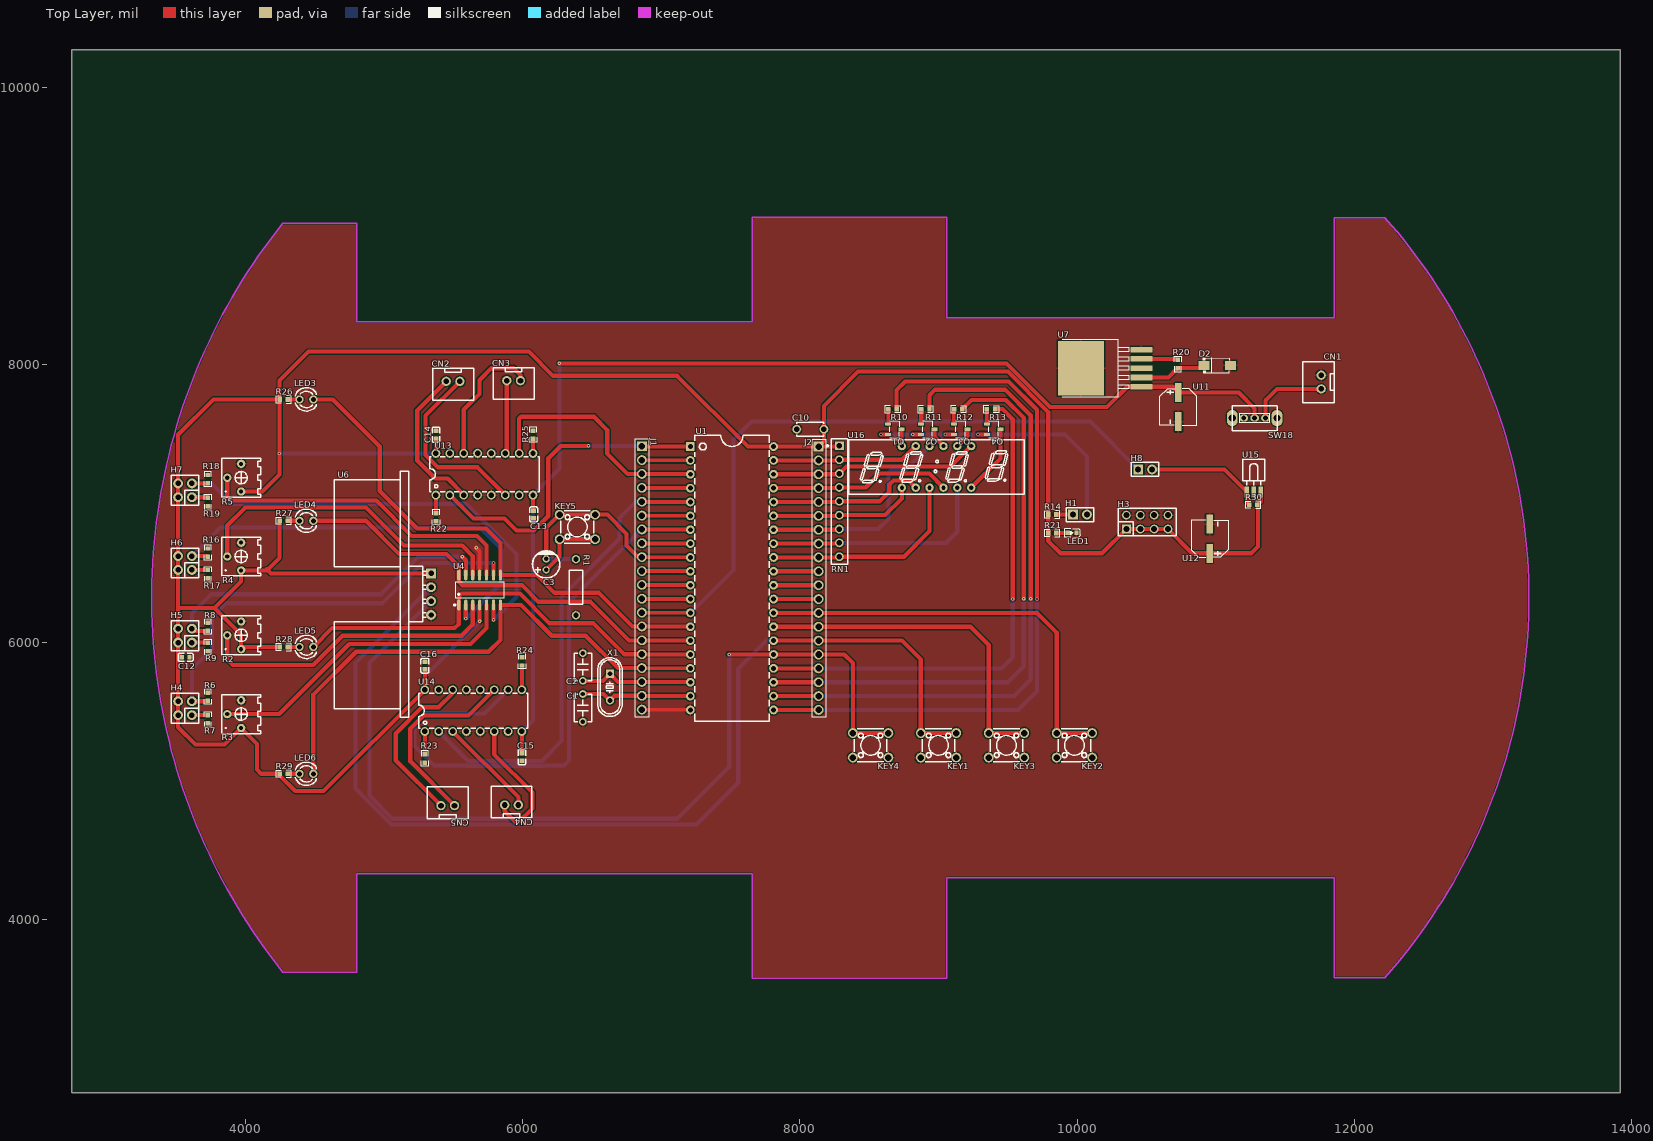
[diagram p0: Top Layer view]
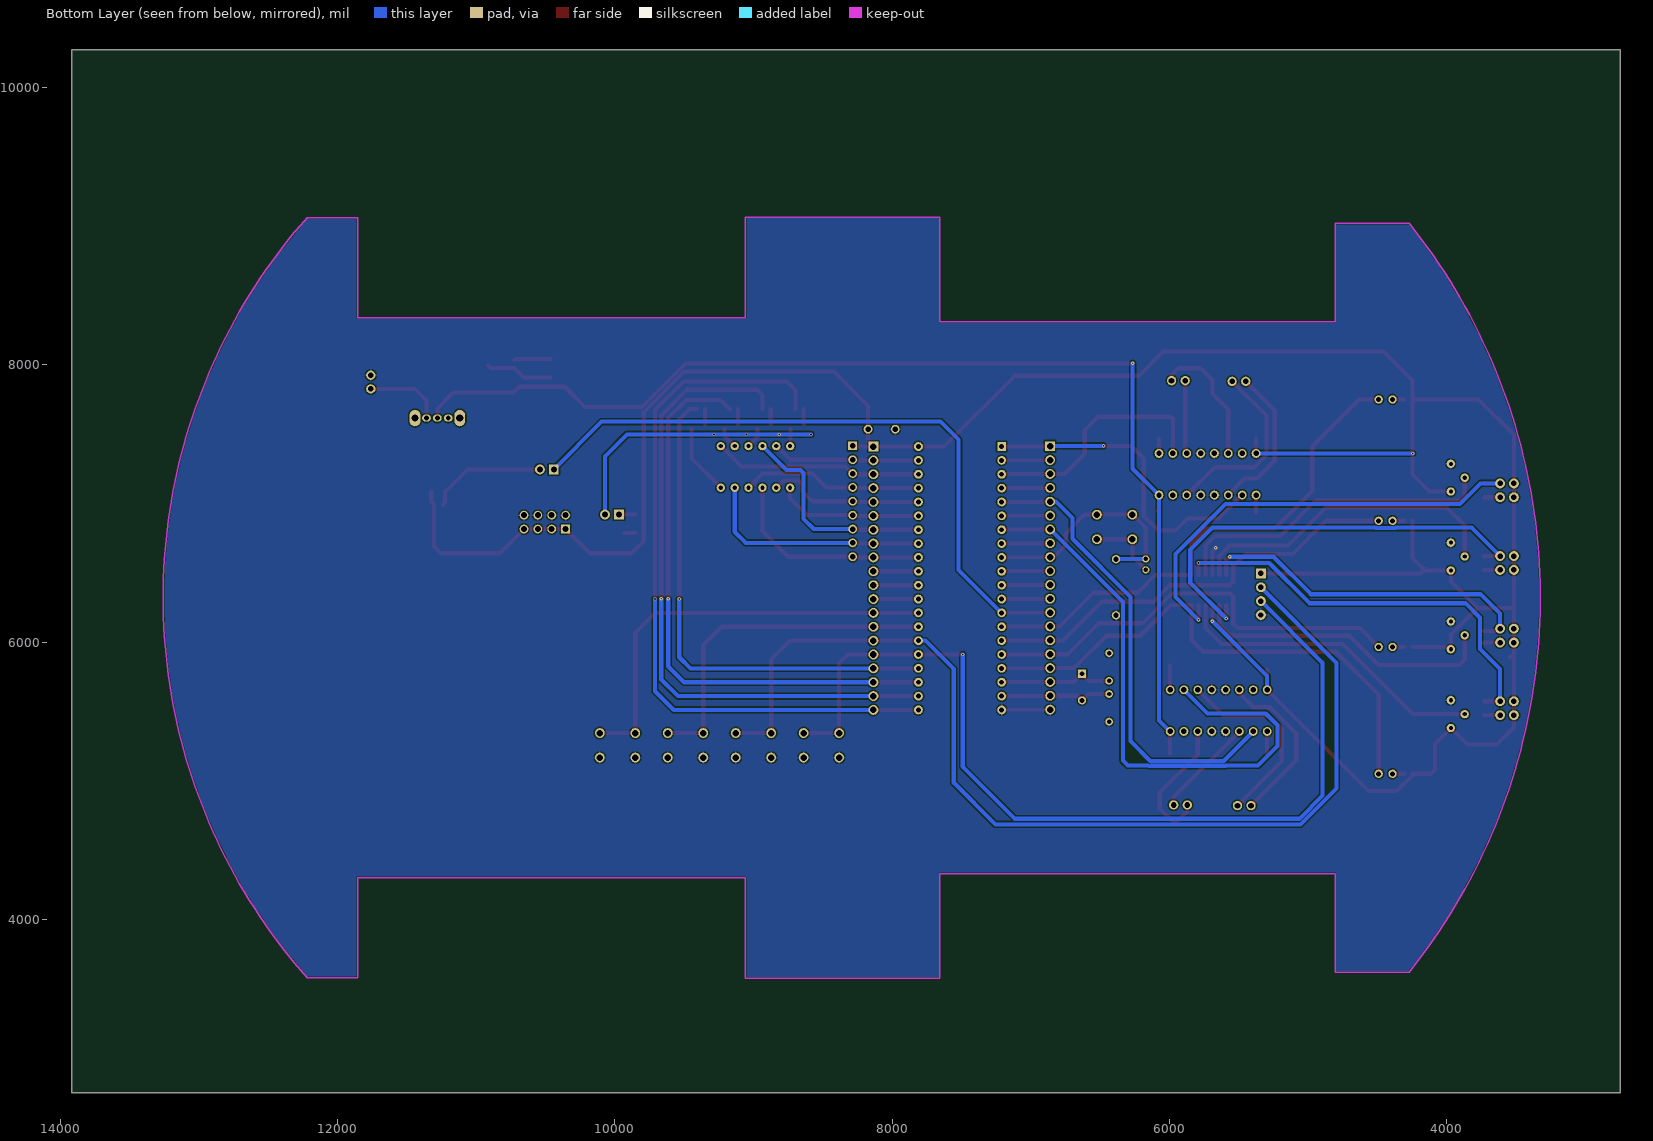
[diagram p1: Bottom Layer view, seen from below]
# Altium PCB MISC51732.pcbdoc
Units mil, origin at the board's own origin, x right, y up, seen from the top; angles counter-clockwise.
Board outline 11165 x 7520 mil, 2 copper layers (Top Layer, Bottom Layer), stack 62.206 mil thick; 80 components, 94 nets, 333 pads, 18 vias.

## Layer stack, top to bottom
Top Solder Mask Layer: solder mask 0.394, Dk 3.3
Top Layer: signal copper 1.379
Dielectric1: surface 59.449, FR4, Dk 4.5
Bottom Layer: signal copper 1.378
Bottom Solder Mask Layer: solder mask 0.394, Dk 3.3

## Board outline
13915,2750 2750,2750 2750,10270 13915,10270

## Design rules (kind name [scope] priority, off if disabled: settings)
BoardOutlineClearance copperThickness2oz_1 [All] p2 off: genericclearance=7.99 ignorepadtopadclearanceinfootprint=FALSE except(0: Arc-SplitContinuation Track-SplitContinuation SMDPad-SplitContinuation THPad-SplitContinuation Via-SplitContinuation Fill-SplitContinuation Region-SplitContinuation Poly-SplitContinuation Text-SplitContinuation Hole-SplitContinuation; 5.98: Arc-CutoutEdge SMDPad-CutoutEdge THPad-CutoutEdge Via-CutoutEdge Fill-CutoutEdge Region-CutoutEdge Text-CutoutEdge; 6.93: Hole-OutlineEdge Hole-CutoutEdge; 10: Poly-OutlineEdge Poly-CutoutEdge; 11.81: Arc-OutlineEdge Track-OutlineEdge SMDPad-OutlineEdge THPad-OutlineEdge Via-OutlineEdge Fill-OutlineEdge Region-OutlineEdge Text-OutlineEdge Track-CutoutEdge)
BoardOutlineClearance copperThickness1oz_1 [All] p4: genericclearance=4.02 ignorepadtopadclearanceinfootprint=FALSE except(0: Arc-SplitContinuation Track-SplitContinuation SMDPad-SplitContinuation THPad-SplitContinuation Via-SplitContinuation Fill-SplitContinuation Region-SplitContinuation Poly-SplitContinuation Text-SplitContinuation Hole-SplitContinuation; 6: SMDPad-CutoutEdge THPad-CutoutEdge Via-CutoutEdge Fill-CutoutEdge Region-CutoutEdge Text-CutoutEdge; 6.93: Hole-OutlineEdge Hole-CutoutEdge; 10: Poly-OutlineEdge Poly-CutoutEdge; 11.8: Arc-OutlineEdge Track-OutlineEdge SMDPad-OutlineEdge THPad-OutlineEdge Via-OutlineEdge Fill-OutlineEdge Region-OutlineEdge Text-OutlineEdge; 11.81: Arc-CutoutEdge Track-CutoutEdge)
Clearance copperThickness2oz [All] p1 off: gap=7.99 ignorepadtopadclearanceinfootprint=FALSE except(5.98: SMDPad-Track SMDPad-SMDPad THPad-Track SMDPad-THPad THPad-THPad Track-Via SMDPad-Via THPad-Via Via-Via Fill-Track Region-Track Fill-SMDPad Region-SMDPad Fill-THPad Region-THPad Fill-Via Region-Via Fill-Fill Fill-Region Region-Region Arc-Track Arc-SMDPad Arc-THPad Arc-Via Fill-Arc Region-Arc Arc-Arc Text-Track SMDPad-Text Text-THPad Text-Via Fill-Text Region-Text Arc-Text Text-Text; 6.93: Hole-Track Hole-SMDPad Hole-THPad Hole-Via Fill-Hole Region-Hole Hole-Arc Hole-Text; 10: Poly-Track Poly-SMDPad Poly-THPad Poly-Via Poly-Fill Poly-Region Poly-Poly Poly-Arc Poly-Text Poly-Hole)
Clearance copperThickness1oz [All] p3: gap=4.02 ignorepadtopadclearanceinfootprint=FALSE except(5.98: SMDPad-Track SMDPad-SMDPad THPad-Track SMDPad-THPad THPad-THPad Track-Via SMDPad-Via THPad-Via Via-Via Fill-Track Region-Track Fill-SMDPad Region-SMDPad Fill-THPad Region-THPad Fill-Via Region-Via Fill-Fill Fill-Region Region-Region; 6: Arc-Track Arc-SMDPad Arc-THPad Arc-Via Fill-Arc Region-Arc Arc-Arc Text-Track SMDPad-Text Text-THPad Text-Via Fill-Text Region-Text Arc-Text Text-Text; 6.93: Hole-Track Hole-SMDPad Hole-THPad Hole-Via Fill-Hole Region-Hole Hole-Arc Hole-Text; 10: Poly-Track Poly-SMDPad Poly-THPad Poly-Via Poly-Fill Poly-Region Poly-Poly Poly-Arc Poly-Text Poly-Hole)
DiffPairsRouting differentialPair [All] p1: maxlimit=6 minlimit=6 mostfreqgap=6 toplayer_minwidth=5 toplayer_prefwidth=10 toplayer_maxwidth=100 toplayer_mingap=6 toplayer_prefgap=6 toplayer_maxgap=6 bottomlayer_minwidth=5 bottomlayer_prefwidth=10 bottomlayer_maxwidth=100 bottomlayer_mingap=6 bottomlayer_prefgap=6 bottomlayer_maxgap=6 maxuncoupledlength=10
HoleToHoleClearance otherClearance [All] p1: gap=11.81 allowstackedmicrovias=TRUE
Length netLength [All] p1: minlimit=0 maxlimit=0
MatchedLengths netLengthTolerance [All] p1: tolerance=1000
PasteMaskExpansion pasteMaskExpansion [All] p1: expansion=0
PlaneConnect innerPlane [All] p1: planeconnectstyle=Relief reliefexpansion=20 reliefentries=4 reliefconductorwidth=10 reliefairgap=10
PolygonConnect copperRegion [(InNet('GND'))] p1: connectstyle=Relief reliefconductorwidth=10 reliefentries=4 polygonreliefangle="90 Angle" airgapwidth=10 via.connectstyle=Relief via.reliefconductorwidth=10 via.reliefentries=4 via.polygonreliefangle="90 Angle" via.airgapwidth=10
RoutingVias viaSize [All] p1: holewidth=12.01 width=24.02 viastyle="Through Hole" minholewidth=11.81 minwidth=19.68 maxholewidth=248.03 maxwidth=393.7
SolderMaskExpansion solderMaskExpansion [IsVia] p1: expansion=-1000 istentingtop=TRUE
SolderMaskExpansion solderMaskExpansion [All] p2: expansion=2 istentingtop=FALSE
Width copperThickness2oz_2 [All] p1 off: maxlimit=100 minlimit=8 preferedwidth=10
Width copperThickness1oz_2 [All] p2: maxlimit=100 minlimit=5 preferedwidth=10

## Components (designator, comment, footprint, x,y, rotation, side; value= is the part's Value field where it differs from the comment)
C1 "" CAP-TH_L5.0-W2.5-P5.08-D0.7 6435,5525 r270 top
C2 "" CAP-TH_L5.0-W2.5-P5.08-D0.7 6435,5820 r90 top
C3 "" CAP-TH_BD5.0-P2.00-D0.8-FD 6170,6560 r90 top
C10 "" CAP-TH_L5.0-W2.5-P5.00-D1.0 8075,7535 r0 top
C12 "104" C0603 3570,5890 r0 top
C13 "100nF" C0603 6080,6920 r270 top
C14 "100nF" C0603 5375,7495 r90 top
C15 "100nF" C0603 5995,5170 r270 top
C16 "100nF" C0603 5295,5830 r90 top
CN1 "XH2.54*2P_through-hole" CONN-TH_2P-P2.50-XH2.54-2P 11760,7875 r270 top
CN2 "XH2.54*2P_through-hole" CONN-TH_2P-P2.50-XH2.54-2P 5498.36,7880.12 r0 top
CN3 "XH2.54*2P_through-hole" CONN-TH_2P-P2.50-XH2.54-2P 5935,7885 r0 top
CN4 "XH2.54*2P_through-hole" CONN-TH_2P-P2.50-XH2.54-2P 5920,4825 r180 top
CN5 "XH2.54*2P_through-hole" CONN-TH_2P-P2.50-XH2.54-2P 5460,4820 r180 top
D2 "SS34" SMA_L4.3-W2.6-LS5.0-RD 11010,7995 r0 top
H1 "" HDR-TH_2P-P2.54-V-M-1 10020.44,6919.23 r0 top
H3 "" HDR-TH_8P-P2.54-V-F-R2-C4-S2.54-1 10505,6865 r0 top
H4 "" HDR-TH_4P-P2.54-V-F-R2-C2-S2.54 3564.9,5522.49 r90 top
H5 "" HDR-TH_4P-P2.54-V-F-R2-C2-S2.54 3564.9,6046.36 r90 top
H6 "" HDR-TH_4P-P2.54-V-F-R2-C2-S2.54 3564.9,6570.23 r90 top
H7 "" HDR-TH_4P-P2.54-V-F-R2-C2-S2.54 3564.9,7094.1 r90 top
H8 "" HDR-TH_2P-P2.54-V-M-1 10490,7245 r0 top
J1 "" HDR-TH_20P-P2.54-V-M-1 6860.16,6462.19 r270 top
J2 "" HDR-TH_20P-P2.54-V-M-1 8135,6460 r270 top
KEY1 "UK-B0202-G5-160" SW-TH_4P-L6.0-W6.0-P4.50-LS6.5 9000,5255 r180 top
KEY2 "UK-B0202-G5-160" SW-TH_4P-L6.0-W6.0-P4.50-LS6.5 9980,5255 r180 top
KEY3 "UK-B0202-G5-160" SW-TH_4P-L6.0-W6.0-P4.50-LS6.5 9490,5255 r180 top
KEY4 "UK-B0202-G5-160" SW-TH_4P-L6.0-W6.0-P4.50-LS6.5 8510,5255 r180 top
KEY5 "UK-B0202-G5-160" SW-TH_4P-L6.0-W6.0-P4.50-LS6.5 6395,6830 r0 top
LED1 "" LED_0603 9961.23,6786.73 r180 top
LED3 "" LED-TH_BD3.0-P2.54-FD 4440.51,7749.41 r0 top
LED4 "" LED-TH_BD3.0-P2.54-FD 4440.51,6874.41 r0 top
LED5 "" LED-TH_BD3.0-P2.54-FD 4440.51,5964.41 r0 top
LED6 "" LED-TH_BD3.0-P2.54-FD 4440.51,5049.41 r0 top
Q1 "S8550" SOT-23-3_L2.9-W1.6-P1.90-LS2.8-BR 8683.19,7534.47 r180 top
Q2 "S8550" SOT-23-3_L2.9-W1.6-P1.90-LS2.8-BR 8921.41,7534.47 r180 top
Q3 "S8550" SOT-23-3_L2.9-W1.6-P1.90-LS2.8-BR 9159.63,7534.47 r180 top
Q4 "S8550" SOT-23-3_L2.9-W1.6-P1.90-LS2.8-BR 9397.84,7534.47 r180 top
R1 "" RES-TH_BD2.4-L6.3-P10.30-D0.6 6385,6395 r270 top
R2 "-" RES-ADJ-TH_3362P 3920,6048.33 r90 top
R3 "-" RES-ADJ-TH_3362P 3920,5480 r90 top
R4 "-" RES-ADJ-TH_3362P 3920,6616.67 r90 top
R5 "-" RES-ADJ-TH_3362P 3920,7185 r90 top
R6 "10K" R0603 3730,5605 r90 top
R7 "100" R0603 3730,5442.91 r270 top
R8 "10K" R0603 3730,6110 r90 top
R9 "100" R0603 3730,5965 r270 top
R10 "1K" R0603 8668.19,7679.47 r180 top
R11 "1K" R0603 8904.89,7679.47 r180 top
R12 "1K" R0603 9141.59,7679.47 r180 top
R13 "1K" R0603 9378.29,7679.47 r180 top
R14 "33" R0603 9820,6920 r0 top
R16 "10K" R0603 3730,6645 r90 top
R17 "100" R0603 3730,6490 r270 top
R18 "10K" R0603 3730,7175 r90 top
R19 "100" R0603 3730,7010 r270 top
R20 "33U" R0603 10725,8005 r270 top
R21 "2K" R0603 9820.46,6786.73 r0 top
R22 "1K" R0603 5375,6900 r90 top
R23 "1K" R0603 5295,5160 r90 top
R24 "1K" R0603 5995,5860 r90 top
R25 "1K" R0603 6075,7495 r90 top
R26 "1K" R0603 4277.03,7749.41 r0 top
R27 "1K" R0603 4277.03,6874.41 r0 top
R28 "1K" R0603 4277.03,5964.41 r0 top
R29 "1K" R0603 4277.03,5049.41 r0 top
R30 "10K" R0603 11270,6990 r0 top
RN1 "" RES-ARRAY-TH_9P-P2.54-D1.0 8285,7015 r270 top
SW18 "" 拨动开关 11285,7615 r180 top
U1 "" DIP-40_L52.0-W13.7-P2.54-LS15.2-BL 7510,6460 r270 top
U4 "LM324NLM324" SOP-14_L8.6-W3.9-P1.27-LS6.0-BL 5690,6375 r0 top
U6 "HC-SR04" TH_HC-SR04V 5340,6345 r270 top
U7 "LM2596SX-5.0/NOPB-YJLTY" TO-263-5_L10.0-W8.4-P1.70-LS15.3-BR 10245,7975 r0 top
U11 "220uF" CAP-SMD_BD6.3-L6.6-W6.6-LS7.2-FD 10730,7695 r270 top
U12 "220uF" CAP-SMD_BD6.3-L6.6-W6.6-LS7.2-FD 10955.02,6745 r90 top
U13 "L293D" DIP-16_L20.0-W6.4-P2.54-LS7.6-BL 5725,7210 r0 top
U14 "L293D" DIP-16_L20.0-W6.4-P2.54-LS7.6-BL 5645,5505 r0 top
U15 "CH0038A_38B/5*5mm/infrared receiver" OPTO-SMD_CH0038A_38B 11273.63,7083.36 r0 top
U16 "0.28 4-digit display" LED-SEG-TH_12P-L32.1-W10.0-P12.7-S7.62-BL 8985.44,7262.93 r0 top
X1 "" HC-49US_L11.5-W4.5-P4.88 6630,5675 r270 top

## Footprints (in the part's own frame and the unit in brackets; to place one, negate y for a bottom-side part, rotate by r counter-clockwise, add the part's x,y. Pads: shape width x height; smd on the part's side, far side on the other; paste and mask are expansions set on the pad)
C0603 [mm]
  rect 0.8x0.9 smd: 1(-0.7,0) 2(0.7,0)
  silkscreen extent -1.39,-0.71 1.39,0.71
CAP-SMD_BD6.3-L6.6-W6.6-LS7.2-FD [mm]
  rect 3.5x1.2 smd: 1(-2.67,0) 2(2.67,0)
  silkscreen extent -3.38,-3.38 3.38,3.38
CAP-TH_BD5.0-P2.00-D0.8-FD [mil]
  round 51.2 hole 31.5 paste+0 mask+2: 1(-39.4,0) 2(39.4,0)
  silkscreen extent -98,-98 98,98
CAP-TH_L5.0-W2.5-P5.00-D1.0 [mil]
  round 63 hole 39.4 paste+0 mask+2: 1(-98.4,0) 2(98.4,0)
  silkscreen extent -98,-50 98,49
CAP-TH_L5.0-W2.5-P5.08-D0.7 [mm]
  round 1.4 hole 0.8 paste+0 mask+0.051: 1(-2.54,0) 2(2.54,0)
  silkscreen extent -2.54,-1.59 2.54,1.59
CONN-TH_2P-P2.50-XH2.54-2P [mm]
  round 1.7 hole 1.05 paste+0 mask+0.05: 1(1.25,0) 2(-1.25,0)
  silkscreen extent -3.75,-3.42 3.75,2.37
DIP-16_L20.0-W6.4-P2.54-LS7.6-BL [mm]
  round 1.6 hole 1: 1(-8.89,-3.81) 2(-6.35,-3.81) 3(-3.81,-3.81) 4(-1.27,-3.81) 5(1.27,-3.81) 6(3.81,-3.81) 7(6.35,-3.81) 8(8.89,-3.81) 9(8.89,3.81) 10(6.35,3.81) 11(3.81,3.81) 12(1.27,3.81) 13(-1.27,3.81) 14(-3.81,3.81) 15(-6.35,3.81) 16(-8.89,3.81)
  silkscreen extent -10,-3.2 10,3.2
DIP-40_L52.0-W13.7-P2.54-LS15.2-BL [mil]
  rect 63x63 hole 35 paste+0 mask+2: 1(-950,-300)
  round 63 hole 35 paste+0 mask+2: 2(-850,-300) 3(-750,-300) 4(-650,-300) 5(-550,-300) 6(-450,-300) 7(-350,-300) 8(-250,-300) 9(-150,-300) 10(-50,-300) 11(50,-300) 12(150,-300) 13(250,-300) 14(350,-300) 15(450,-300) 16(550,-300) 17(650,-300) 18(750,-300) 19(850,-300) 20(950,-300) 21(950,300) 22(850,300) 23(750,300) 24(650,300) 25(550,300) 26(450,300) 27(350,300) 28(250,300) 29(150,300) 30(50,300) 31(-50,300) 32(-150,300) 33(-250,300) 34(-350,300) 35(-450,300) 36(-550,300) 37(-650,300) 38(-750,300) 39(-850,300) 40(-950,300)
  silkscreen extent -1030,-270 1030,270
HC-49US_L11.5-W4.5-P4.88 [mil]
  rect 59.1x59.1 hole 35.4 paste+0 mask+2: 1(-96.1,0)
  round 59.1 hole 35.4 paste+0 mask+2: 2(96.1,0)
  silkscreen extent -212,-89 212,89
HDR-TH_2P-P2.54-V-M-1 [mm]
  rect 1.8x1.8 hole 1.1: 1(-1.27,0)
  round 1.8 hole 1.1: 2(1.27,0)
  silkscreen extent -2.54,-1.27 2.54,1.27
HDR-TH_4P-P2.54-V-F-R2-C2-S2.54 [mm]
  round 1.8 hole 1: 1(-1.27,-1.27) 2(-1.27,1.27) 3(1.27,-1.27) 4(1.27,1.27)
  silkscreen extent -2.74,-2.5 2.74,2.5
HDR-TH_8P-P2.54-V-F-R2-C4-S2.54-1 [mm]
  rect 1.6x1.6 hole 1.1: 1(-3.81,-1.27)
  round 1.6 hole 1.1: 2(-3.81,1.27) 3(-1.27,-1.27) 4(-1.27,1.27) 5(1.27,-1.27) 6(1.27,1.27) 7(3.81,-1.27) 8(3.81,1.27)
  silkscreen extent -5.28,-2.5 5.28,2.5
HDR-TH_20P-P2.54-V-M-1 [mil]
  rect 70.9x70.9 hole 47.2 paste+0 mask+2: 1(-950,0)
  round 70.9 hole 47.2 paste+0 mask+2: 2(-850,0) 3(-750,0) 4(-650,0) 5(-550,0) 6(-450,0) 7(-350,0) 8(-250,0) 9(-150,0) 10(-50,0) 11(50,0) 12(150,0) 13(250,0) 14(350,0) 15(450,0) 16(550,0) 17(650,0) 18(750,0) 19(850,0) 20(950,0)
  silkscreen extent -1000,-50 1000,55
LED-SEG-TH_12P-L32.1-W10.0-P12.7-S7.62-BL [mil]
  round 60 hole 30: 1(-250,-150) 2(-150,-150) 3(-50,-150) 4(50,-150) 5(150,-150) 6(250,-150) 7(250,150) 8(150,150) 9(50,150) 10(-50,150) 11(-150,150) 12(-250,150)
  silkscreen extent -634,-197 634,197
LED-TH_BD3.0-P2.54-FD [mil]
  round 60 hole 36 paste+0 mask+2: 1(-50,0) 2(50,0)
  silkscreen extent -81,-84 72,85
LED_0603 [mil]
  rect 31.5x31.5 smd paste+0 mask+2: 1(-33.5,-0.4) 2(29.5,-0.2)
  silkscreen extent -61,-30 53,30
OPTO-SMD_CH0038A_38B [mm]
  rect 0.8x2 smd paste+0 mask+0.05: 1(-1.27,0) 2(0,0) 3(1.27,0)
  silkscreen extent -2,1.23 2,6
R0603 [mil]
  rect 31.75x34.02 smd paste-3937.01 mask+2: 1(-29.66,0) 2(29.66,0)
  silkscreen extent -55,-26 55,26
RES-ADJ-TH_3362P [mil]
  round 60 hole 30: 1(-100,-50) 2(0,50) 3(100,-50)
  silkscreen extent -140,-190 140,90
RES-ARRAY-TH_9P-P2.54-D1.0 [mm]
  rect 1.6x1.6 hole 1 paste+0 mask+0.051: 1(-10.16,0)
  round 1.6 hole 1 paste+0 mask+0.051: 2(-7.62,0) 3(-5.08,0) 4(-2.54,0) 5(0,0) 6(2.54,0) 7(5.08,0) 8(7.62,0) 9(10.16,0)
  silkscreen extent -11.5,-2.31 11.5,1.5
RES-TH_BD2.4-L6.3-P10.30-D0.6 [mil]
  round 60 hole 39.37 paste+0 mask+2: 1(-202.76,0) 2(202.76,0)
  silkscreen extent -124,-47 124,47
SMA_L4.3-W2.6-LS5.0-RD [mm]
  rect 2.046x1.62 smd: 1(-2.404,-0.009) 2(2.404,0.009)
  silkscreen extent -2.61,-1.44 2.16,1.44
SOP-14_L8.6-W3.9-P1.27-LS6.0-BL [mm]
  oval 0.595x1.968 smd: 1(-3.81,-2.734) 2(-2.54,-2.734) 3(-1.27,-2.734) 4(0,-2.734) 5(1.27,-2.734) 6(2.54,-2.734) 7(3.81,-2.734) 8(3.81,2.734) 9(2.54,2.734) 10(1.27,2.734) 11(0,2.734) 12(-1.27,2.734) 13(-2.54,2.734) 14(-3.81,2.734)
  silkscreen extent -4.71,-2.88 4.4,1.52
SOT-23-3_L2.9-W1.6-P1.90-LS2.8-BR [mm]
  rect 1.07x0.6 smd: 1(1.235,-0.95) 2(1.235,0.95) 3(-1.235,0)
  silkscreen extent -0.88,-1.54 0.88,1.54
SW-TH_4P-L6.0-W6.0-P4.50-LS6.5 [mm]
  round 1.8 hole 1.2 paste+0 mask+0.051: 1(-3.25,2.25) 2(3.25,2.25) 3(-3.25,-2.25) 4(3.25,-2.25)
  silkscreen extent -3,-3 3,3
TH_HC-SR04V [mm]
  rect 1.8x1.8 hole 1.001: 1(-3.81,0)
  round 1.8 hole 1.001: 2(-1.27,0) 3(1.27,0) 4(3.81,0)
  silkscreen extent -22.5,-17.7 22.5,-0.89
TO-263-5_L10.0-W8.4-P1.70-LS15.3-BR [mm]
  rect 4x1.02 smd: 1(5.55,-3.4) 2(5.55,-1.7) 3(5.55,0) 4(5.55,1.7) 5(5.55,3.4)
  rect 8.4x10 smd: 6(-5.55,0)
  silkscreen extent -8.91,-5.33 3.2,5.33
拨动开关 [mil]
  oval 63x51.2 hole 35.4 paste+0 mask+2: 1(-73.4,0) 2(5,0) 3(84,0)
  oval 78.7x118.1 hole 51.2 paste+0 mask+2: 4(166.7,0) 5(-156.1,0)
  silkscreen extent -156,-90 167,90

## Via types
v1: diameter 24.02, hole 12, Top Layer to Bottom Layer, 18 vias

## Nets (pads, with @x,y where several pads share a name; then routed paths per layer and width w, separated by ;. In a path a pad name is that pad's centre, name@x,y a point inside that pad or via, vN(x,y) a via of type N, cw(c..) or ccw(c..) an arc to the next point about the centre after c; other vN are vias at no path point)
7.2V: C13.1 C15.1 SW18.2 U7.1 U11.1 U13.8 U14.8 | length 8379.5
  Top Layer w30: C15.1 U14.8 ; U13.8 6075,6952.56 C13.1 ; v1(6265,8010) 9490,8010 9805,7695 10215,7695 10361.14,7841.14 U7.1 10688.97,7841.14 U11.1 11164.88,7800.12 11280,7685 SW18.2
  Bottom Layer w30: U14.8 6075,5435 U13.8 6265,7250 v1(6265,8010)
$1N43: J2.11 U1.30 | length 325
  Top Layer w30: U1.30 J2.11
$1N44: J2.12 U1.29 | length 325
  Top Layer w30: U1.29 J2.12
$1N233: H4.1 R7.1 | length 115.1
  Top Layer w30: H4.1 3729.91,5472.49 R7.1
$1N236: H5.1 R9.1 | length 115.8
  Top Layer w30: H5.1 3728.3,5996.36 R9.1
$1N238: H6.1 R17.1 | length 115.3
  Top Layer w30: H6.1 3729.43,6520.23 R17.1
$1N240: H7.1 R19.1 | length 116.9
  Top Layer w30: H7.1 3725.56,7044.1 R19.1
$1N251: D2.1 R20.2 U7.2 | length 487.7
  Top Layer w30: U7.2 10657.73,7908.07 R20.2 10896.07,7975.34 D2.1
$1N255: CN1.1 SW18.1 | length 564.1
  Top Layer w30: SW18.1 11358.4,7743.4 11440.78,7825.78 CN1.1
$1N261: LED1.2 R21.2 | length 81.7
  Top Layer w30: R21.2 9850.32,6786.93 LED1.2
$1N276: R22.2 U13.1 | length 130.3
  Top Layer w30: R22.2 U13.1
$1N301: R23.2 U14.1 | length 165.3
  Top Layer w30: R23.2 U14.1
$1N314: R24.1 U14.9 | length 175.3
  Top Layer w30: U14.9 R24.1
$1N316: R25.1 U13.9 | length 105.3
  Top Layer w30: U13.9 R25.1
$1N318: LED3.1 R26.2 | length 83.8
  Top Layer w30: R26.2 LED3.1
$1N319: LED4.1 R27.2 | length 83.8
  Top Layer w30: R27.2 LED4.1
$1N320: LED5.1 R28.2 | length 83.8
  Top Layer w30: R28.2 LED5.1
$1N321: LED6.1 R29.2 | length 83.8
  Top Layer w30: R29.2 LED6.1
$1N330: H8.2 R30.1 U15.1 | length 850.9
  Top Layer w30: H8.2 11061.99,7245 U15.1 11223.63,7006.71 R30.1
$1N340: Q1.3 U16.12 | length 123
  Top Layer w30: Q1.3 8731.82,7416.56 U16.12
$1N341: Q1.1 R10.2 | length 109.2
  Top Layer w30: Q1.1 8638.53,7575.84 R10.2
$1N342: H1.2 Q1.2 Q2.2 Q3.2 Q4.2 | length 2203.6
  Top Layer w30: v1(8585,7497.07) Q1.2 ; v1(8815,7497.07) Q2.2 ; v1(9050,7497.07) Q3.2 ; v1(9285,7497.07) Q4.2
  Bottom Layer w30: v1(8585,7497.07) v1(8815,7497.07) v1(9050,7497.07) v1(9285,7497.07) 9912.93,7497.07 10070.44,7339.56 H1.2
$1N344: Q2.3 U16.9 | length 148.6
  Top Layer w30: Q2.3 8970.04,7478.34 U16.9
$1N345: Q2.1 R11.2 | length 108.6
  Top Layer w30: Q2.1 8875.23,7574.32 R11.2
$1N347: Q3.3 U16.8 | length 151.7
  Top Layer w30: U16.8 9208.25,7485.74 Q3.3
$1N348: Q3.1 R12.2 | length 108
  Top Layer w30: Q3.1 9111.93,7572.8 R12.2
$1N350: Q4.3 U16.6 | length 508.9
  Top Layer w30: U16.6 9446.47,7323.96 Q4.3
$1N351: Q4.1 R13.2 | length 107.8
  Top Layer w30: R13.2 9348.63,7572.46 Q4.1
$1N356: H1.1 R14.2 | length 121.1
  Top Layer w30: R14.2 9850.43,6919.23 H1.1
+5V: C3.1 KEY5.3 KEY5.4 | length 516.9
  Top Layer w30: C3.1 6267.05,6617.65 KEY5.3 KEY5.4
EA: J2.10 U1.31 | length 325
  Top Layer w30: U1.31 J2.10
EN1: R22.1
EN2: R25.2
EN3: R23.1
EN4: R24.2
GND: C1.2 C2.2 C10.1 C12.2 C13.2 C14.2 C15.2 C16.2 CN1.2 D2.2 H3.2 H3.4 H3.6 H3.8 J1.20 KEY1.1 KEY1.2 KEY2.1 KEY2.2 KEY3.1 KEY3.2 KEY4.1 KEY4.2 LED1.1 R1.2 R2.3 R3.3 R4.3 R5.3 R6.2 R7.2 R8.2 R9.2 R16.2 R17.2 R18.2 R19.2 U1.20 U4.11 U6.4 U7.5 U7.6 U11.2 U12.2 U13.4 U13.5 U13.12 U13.13 U14.4 U14.5 U14.12 U14.13 U15.2 | length 557.6
  Top Layer w30: v1(5665,6680) 5690,6655 U4.11 ; J1.20 U1.20
IN1: J1.1 U1.1 U13.2 | length 2337.6
  Top Layer w30: U13.2 5645,6890 5870,6890 5955,6805 6080,6805 6185,6910 6185,7325 6275,7415 v1(6475,7415) ; J1.1 U1.1
  Bottom Layer w30: v1(6475,7415) 6857.35,7415 J1.1
IN2: U13.7
IN3: J1.3 U1.3 U13.10 | length 1761.8
  Top Layer w30: U13.10 5975,7610 5990,7625 6515,7625 6610,7530 6610,7360 6757.81,7212.19 J1.3 U1.3
IN4: U13.15
IN5: J1.5 U1.5 U14.2 | length 3376.6
  Top Layer w30: J1.5 U1.5
  Bottom Layer w30: U14.2 5610,5140 6135,5140 6280,5285 6280,6325 6700,6745 6700,6895 6817.19,7012.19 J1.5
IN6: U14.7
IN7: J1.7 U1.7 U14.10 | length 4358.6
  Top Layer w30: J1.7 U1.7
  Bottom Layer w30: U14.10 5725,5485 5305,5485 5220,5400 5220,5250 5360,5110 5591.89,5110 5595.91,5105.98 6149.09,5105.98 6153.11,5110 6300,5110 6335,5145 6335,6170.14 6334.02,6171.12 6334.02,6213.36 6335,6214.34 6335,6290 6857.19,6812.19 J1.7
IN8: U14.15
OUT1: CN2.2 U13.3 | length 1098.2
  Top Layer w30: CN2.2 5240,7670.97 5240,7310 5370,7180 5460,7180 5575,7065 U13.3
OUT2: CN2.1 U13.6 | length 1327.8
  Top Layer w30: CN2.1 5300,7632.54 5300,7350 5390,7260 5675,7260 U13.6
OUT3: CN3.2 U13.11 | length 529.5
  Top Layer w30: U13.11 5885.78,7370.78 CN3.2
OUT4: CN3.1 U13.14 | length 968.2
  Top Layer w30: U13.14 5575,7675 5688.01,7788.01 5688.01,7888.01 5775,7975 5935,7975 5984.22,7925.78 CN3.1
OUT5: CN4.2 U14.3 | length 726.4
  Top Layer w30: U14.3 5969.22,4880.78 CN4.2
OUT6: CN4.1 U14.6 | length 984
  Top Layer w30: U14.6 5795,5190 6070,4915 6070,4800 5975,4705 5945,4705 5870.78,4779.22 CN4.1
OUT7: CN5.2 U14.11 | length 1408.2
  Top Layer w30: CN5.2 5509.22,4820.78 5190,5140 5190,5375 5285,5470 5610,5470 U14.11
OUT8: CN5.1 U14.14 | length 1210.1
  Top Layer w30: CN5.1 5085,5145.78 5085,5340 5275,5530 5395,5530 5495,5630 U14.14
OV1: R5.2 U4.10 | length 2364.4
  Top Layer w30: R5.2 3870,7050 3900,7020 4945,7020 5200,6765 5670,6765 5740,6695 U4.10
OV2: R4.2 U4.12 | length 2329.5
  Top Layer w30: R4.2 3870,6840 4000,6970 4870,6970 5145,6695 5565,6695 5640,6620 U4.12
OV3: R2.2 U4.3 | length 2222.4
  Top Layer w30: R2.2 3870,5875 3910,5835 4490,5835 4700,6045 5560,6045 5640,6125 U4.3
OV4: R3.2 U4.5 | length 2294.2
  Top Layer w30: R3.2 4245,5480 4750,5985 5625,5985 5740,6100 U4.5
P0.0: J2.2 RN1.2 U1.39 U16.11 | length 1067.3
  Top Layer w30: U1.39 J2.2 8272.93,7310 ccw(c8272.93,7327.07) RN1.2 8737.51,7315 U16.11
P0.1: J2.3 RN1.3 U1.38 U16.7 | length 1508.8
  Top Layer w30: U1.38 J2.3 8272.93,7210 ccw(c8272.93,7227.07) RN1.3 8335,7265 9087.51,7265 U16.7
P0.2: J2.4 RN1.4 U1.37 U16.4 | length 1310.5
  Top Layer w30: U1.37 J2.4 8272.93,7110 ccw(c8272.93,7127.07) RN1.4 8475,7115 8575,7215 8933.38,7215 U16.4
P0.3: J2.5 RN1.5 U1.36 U16.2 | length 1139.8
  Top Layer w30: U1.36 J2.5 8272.93,7010 ccw(c8272.93,7027.07) RN1.5 8575,7015 8645,7085 8645,7135 8675,7165 8783.38,7165 U16.2
P0.4: J2.6 RN1.6 U1.35 U16.1 | length 1054.2
  Top Layer w30: U1.35 J2.6 8272.93,6910 ccw(c8272.93,6927.07) RN1.6 8615,6915 8735.44,7035.44 U16.1
P0.5: J2.7 RN1.7 U1.34 U16.10 | length 1567.8
  Top Layer w30: U1.34 J2.7 8272.93,6810 ccw(c8272.93,6827.07) RN1.7
  Bottom Layer w30: RN1.7 8565,6815 8638.79,6888.79 8638.79,7218.79 8660,7240 8762.51,7240 U16.10
P0.6: J2.8 RN1.8 U1.33 U16.5 | length 1677.6
  Top Layer w30: U1.33 J2.8 8272.93,6710 ccw(c8272.93,6727.07) RN1.8
  Bottom Layer w30: RN1.8 9055,6715 9135.44,6795.44 U16.5
P0.7: J2.9 RN1.9 U1.32 U16.3 | length 1516.1
  Top Layer w30: U1.32 J2.9 8272.93,6610 ccw(c8272.93,6627.07) RN1.9 8750,6615 8935.44,6800.44 U16.3
P1.1: J1.2 U1.2 | length 349.8
  Top Layer w30: J1.2 U1.2
P1.3: J1.4 U1.4 | length 349.8
  Top Layer w30: J1.4 U1.4
P1.5: J1.6 U1.6 | length 349.8
  Top Layer w30: J1.6 U1.6
P1.7: J1.8 U1.8 | length 349.8
  Top Layer w30: J1.8 U1.8
P2.0: J2.20 R10.1 U1.21 | length 5247.1
  Top Layer w30: U1.21 J2.20 ; R10.1 8697.85,7817.85 8760,7880 9505,7880 9710,7675 v1(9710,6310.02)
  Bottom Layer w30: J2.20 9575,5510 9710,5645 v1(9710,6310.02)
P2.1: J2.19 R11.1 U1.22 | length 4733.6
  Top Layer w30: U1.22 J2.19 ; R11.1 8935,7679.92 8935,7780 8975,7820 9480,7820 9665,7635 v1(9665,6311.08)
  Bottom Layer w30: J2.19 9545,5610 9665,5730 v1(9665,6311.08)
P2.2: J2.18 R12.1 U1.23 | length 4167.4
  Top Layer w30: U1.23 J2.18 ; R12.1 9236.78,7745 9485,7745 9615,7615 v1(9615,6311.08)
  Bottom Layer w30: J2.18 9500,5710 9615,5825 v1(9615,6311.08)
P2.3: J2.17 R13.1 U1.24 | length 3631
  Top Layer w30: U1.24 J2.17 ; R13.1 9460.53,7679.47 9535,7605 v1(9535,6310)
  Bottom Layer w30: J2.17 9455,5810 9535,5890 v1(9535,6310)
P2.4: J2.16 KEY4.3 KEY4.4 U1.25 U6.3 | length 6894.2
  Top Layer w30: v1(7490,5910) U1.25 J2.16 8320,5910 8382.05,5847.95 KEY4.4 KEY4.3
  Bottom Layer w30: U6.3 4895,5850 4895,4893.11 5063.11,4725 7115,4725 7490,5100 v1(7490,5910)
P2.5: J2.15 KEY1.3 KEY1.4 U1.26 U6.2 | length 7731.7
  Top Layer w30: U1.26 J2.15 8735,6010 8872.05,5872.95 KEY1.4 KEY1.3
  Bottom Layer w30: U6.2 4795,5850 4795,4945 5055,4685 7255,4685 7555,4985 7555,5805 7760,6010 U1.26
P2.6: J2.14 KEY3.3 KEY3.4 U1.27 | length 2497
  Top Layer w30: U1.27 J2.14 9230,6110 9362.05,5977.95 KEY3.4 KEY3.3
P2.7: J2.13 KEY2.3 KEY2.4 U1.28 | length 3081.2
  Top Layer w30: U1.28 J2.13 9710,6210 9852.05,6067.95 KEY2.4 KEY2.3
P3.0: J1.10 U1.10 | length 349.8
  Top Layer w30: J1.10 U1.10
P3.1: J1.11 U1.11 | length 349.8
  Top Layer w30: J1.11 U1.11
P3.2: J1.12 U1.12 | length 349.8
  Top Layer w30: J1.12 U1.12
P3.3: H8.1 J1.13 U1.13 | length 4845
  Top Layer w30: J1.13 U1.13
  Bottom Layer w30: U1.13 7520,6520 7520,7460 7650,7590 10095,7590 H8.1
P3.4: J1.14 LED3.2 U1.14 U4.8 | length 3721.2
  Top Layer w30: LED3.2 4630.59,7749.41 4970,7410 4970,7090 5240,6820 5735,6820 5840,6715 U4.8 6102.37,6482.63 6230,6355 6550,6355 6792.81,6112.19 J1.14 U1.14
P3.5: J1.15 LED4.2 U1.15 U4.14 | length 3141.1
  Top Layer w30: LED4.2 4870.59,6874.41 5110,6635 5450,6635 5540,6545 U4.14 5540,6435 5565,6410 5995,6410 6115,6290 6490,6290 6767.81,6012.19 J1.15 U1.15
P3.6: J1.16 LED5.2 U1.16 U4.1 | length 3177.7
  Top Layer w30: LED5.2 4626.1,6100 5510,6100 5540,6130 U4.1 5540,6330 5560,6350 5980,6350 6195,6135 6510,6135 6732.81,5912.19 J1.16 U1.16
P3.7: J1.17 LED6.2 U1.17 U4.7 | length 3894.9
  Top Layer w30: LED6.2 4490.51,5620.51 4800,5930 5755,5930 5840,6015 U4.7 5987.63,6267.37 6210,6045 6455,6045 6687.81,5812.19 J1.17 U1.17
RST: C3.2 J1.9 KEY5.1 KEY5.2 R1.1 U1.9 | length 1694.7
  Top Layer w30: C3.2 6170,6821.53 KEY5.1 KEY5.2 6611.42,6918.58 6750,6780 6750,6695 6832.81,6612.19 J1.9 U1.9
  Bottom Layer w30: C3.2 6383.36,6599.4 R1.1
S$164: 
VCC: C10.2 C12.1 C14.1 C16.1 H3.1 H3.3 H3.5 H3.7 H4.2 H4.4 H5.2 H5.4 H6.2 H6.4 H7.2 H7.4 J2.1 R2.1 R3.1 R4.1 R5.1 R14.1 R21.1 R26.1 R27.1 R28.1 R29.1 R30.2 RN1.1 U1.40 U4.4 U6.1 U12.1 U13.16 U14.16 U15.3 | length 21301.7
  Top Layer w30: C12.1 3533.67,5898.77 3514.9,5898.77 ; R5.1 4125,7085 4247.37,7207.37 R26.1 ; 4155,6525 4160,6520 ; R28.1 3986.07,5964.41 R2.1 3970,6055 3778.86,6246.14 ; R27.1 4247.37,6607.37 4160,6520 ; C16.1 U14.16 4565,4925 4360,4925 4247.37,5037.63 R29.1 4115,5049.41 4085,5079.41 4085,5265 R3.1 3850,5260 3640,5260 3514.9,5385.1 H4.2 H4.4 3514.9,5898.77 ; U6.1 4185,6495 4160,6520 ; U13.16 C14.1 ; v1(5690,6150) U4.4 ; RN1.1 8280,7410 J2.1 ; R14.1 R14.1@9790.8,6919.54 ; U15.3 11323.63,7013.97 R30.2 11305,6984.66 11305,6690 11254.89,6639.89 U12.1 10830.11,6639.89 H3.7 H3.5 H3.3 H3.1 10180,6640 9880,6640 9790.8,6729.2 R21.1 R14.1@9790.8,6919.54 ; 3514.9,5898.77 H5.2 H5.4 3514.9,6246.14 ; 3514.9,6246.14 3778.86,6246.14 ; 3514.9,6246.14 H6.2 H6.4 H7.2 H7.4 3514.9,7494.66 cw(c7611.59,6331.47) 3514.99,7494.99 3769.41,7749.41 R26.1 ; 3778.86,6246.14 3970,6437.27 R4.1 4156.67,6516.67 4160,6520 ; R26.1 4247.37,7887.37 4455,8095 6045,8095 6220,7920 7115,7920 7625,7410 U1.40 J2.1 ; J2.1 8173.4,7448.4 C10.2 8173.4,7703.4 8420,7950 9500,7950 9790.8,7659.2 R14.1@9790.8,6919.54
  Bottom Layer w30: v1(4245,7360) U13.16 ; U14.16 5295,5755 v1(5690,6150)
VCC-5: R20.1 U7.4 | length 264.5
  Top Layer w30: U7.4 10717.73,8041.93 R20.1
XIN1: H4.3 R6.1 U4.9 | length 3059.9
  Top Layer w30: H4.3 3727.15,5572.49 R6.1 ; U4.9 v1(5790,6570)
  Bottom Layer w30: H4.3 3614.9,5804.9 3760,5950 3760,6175 3865,6280 4990,6280 5280,6570 v1(5790,6570)
XIN2: H5.3 R8.1 U4.13 | length 2493
  Top Layer w30: H5.3 3630.91,6080.34 R8.1 ; v1(5565,6615) 5590,6590 U4.13
  Bottom Layer w30: H5.3 3614.9,6204.9 3755,6345 4980,6345 5250,6615 v1(5565,6615)
XIN3: H6.3 R16.1 U4.2 | length 3204.7
  Top Layer w30: H6.3 3725.11,6620.23 R16.1 ; v1(5590,6170) U4.2
  Bottom Layer w30: H6.3 3819.67,6825 4367.81,6825 4369.39,6823.42 4511.62,6823.42 4513.2,6825 5690,6825 5850,6665 5850,6430 v1(5590,6170)
XIN4: H7.3 R18.1 U4.6 | length 3317.3
  Top Layer w30: H7.3 3728.76,7144.1 R18.1 ; v1(5790,6160) U4.6
  Bottom Layer w30: H7.3 3755.9,7144.1 3905,6995 5595,6995 5955,6635 5955,6325 v1(5790,6160)
XTAL1: C1.1 J1.19 U1.19 X1.2 | length 807.9
  Top Layer w30: C1.1 6583.9,5625 X1.2 6663.29,5612.19 J1.19 U1.19
XTAL2: C2.1 J1.18 U1.18 X1.1 | length 820.6
  Top Layer w30: C2.1 6578.9,5720 X1.1 6688.91,5712.19 J1.18 U1.18
pads on no net: SW18.3 SW18.4 SW18.5 U7.3

## Polygon pours and split planes (outlines as drawn)
GND on Top Layer (solid, remove dead copper, pour order 0): 3000,10020 3000,3000 13665,3000 13665,10020
GND on Bottom Layer (solid, remove dead copper, pour order 2): 3060,9910 3060,3130 13510,3130 13510,9910

## Keep-outs
Board Outline Layer:
  lines w10: 4270,3620 cw(c7652.79,6320) 4270,9020 4805,9020 4805,8310 7655,8310 7655,9065 9060,9065 9060,8340 11855,8340 11855,9060 12220,9060 cw(c9121.78,6320) 12220,3580 11855,3580 11855,4300 9060,4300 9060,3575 7655,3575 7655,4330 4805,4330 4805,3620 4270,3620